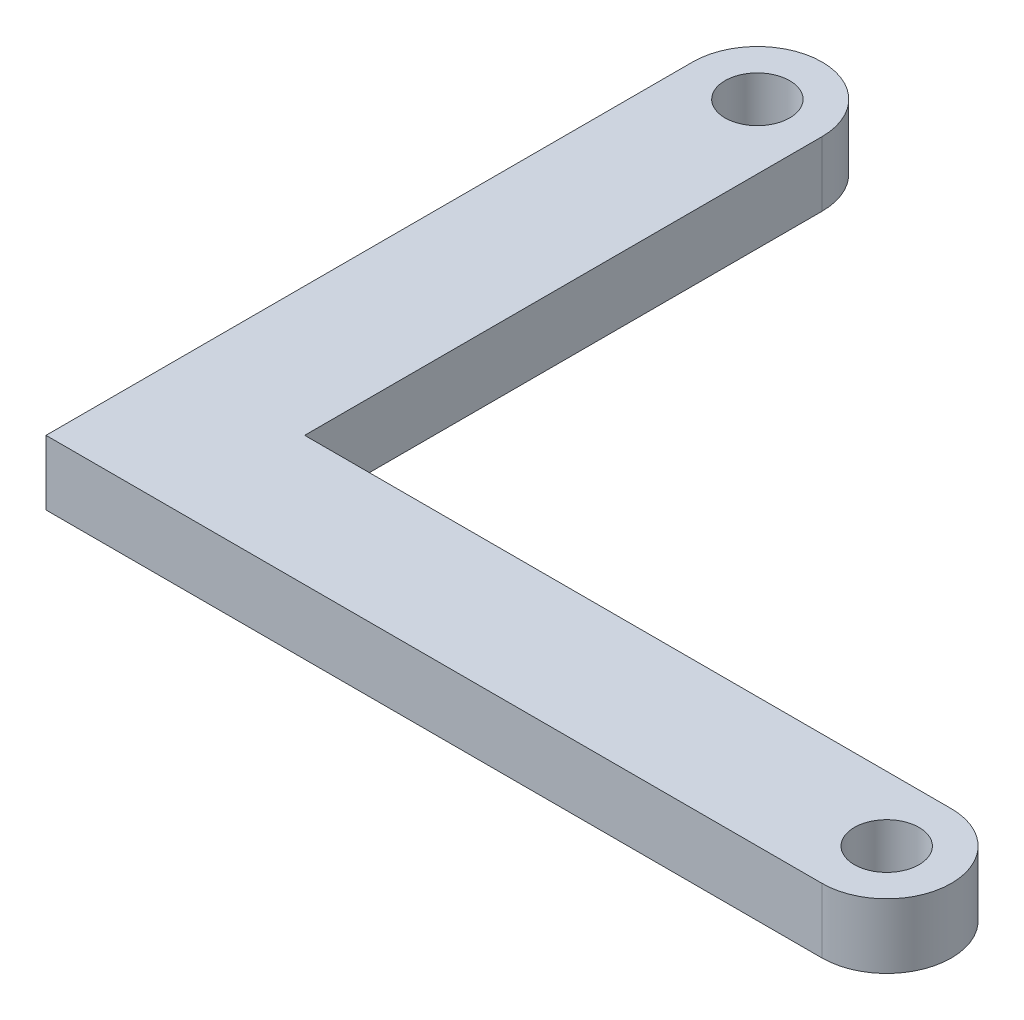
SolidWorks part; units mm, degrees
ref_plane "Front Plane" through (0, 0, 0) normal (0, 0, 1) x (1, 0, 0)
ref_plane "Top Plane" through (0, 0, 0) normal (0, 1, 0) x (1, 0, 0)
ref_plane "Right Plane" through (0, 0, 0) normal (1, 0, 0) x (0, 0, -1)
sketch "Sketch1" plane through (0, 0, 0) normal (0, 1, 0) x (1, 0, 0)
  line L1 (-25, -5) -> (25, -5)
  line L3 (-25, 5) -> (25, 5)
  line L7 (-25, -5) -> (-35, -5)
  line L8 (-25, 5) -> (-25, 45)
  line L10 (-35, -5) -> (-35, 45)
  arc A0 (25, -5) -> (25, 5) centre (25, 0) ccw
  circle A1 centre (25, 0) radius 2.5
  arc A2 (-25, 45) -> (-35, 45) centre (-30, 45) ccw
  circle A3 centre (-30, 45) radius 2.5
  point P0 (0, 0)
  dimension "D5" = 5
  dimension "D6" = 5
  dimension "D1" = 50
  dimension "D2" = 10
  dimension "D3" = 50
  dimension "D4" = 10
extrude "Boss-Extrude1" add sketch "Sketch1" along normal blind 5
